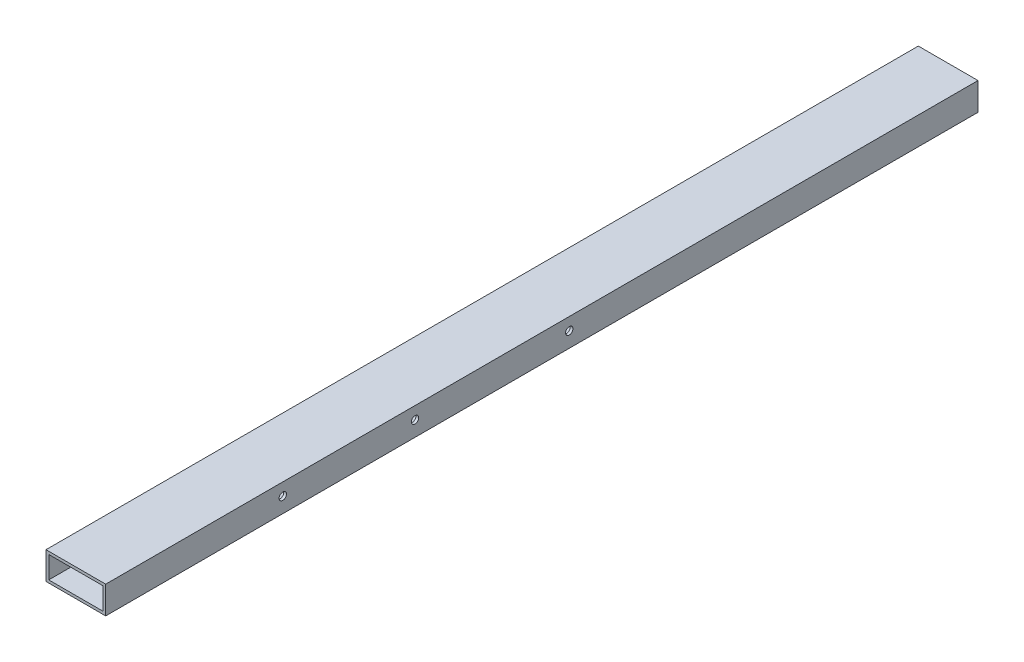
from build123d import *

# Parameters (mm, degrees)
SKETCH1_W           = 65
SKETCH1_H           = 30
BOSS_EXTRUDE1_DEPTH = 950
SKETCH2_W           = 59
SKETCH2_H           = 24
CUT_EXTRUDE1_DEPTH  = 950
SKETCH5_R           = 4
CUT_EXTRUDE2_DEPTH  = 954.05282071


with BuildPart() as part:
    # Sketch1 → Boss-Extrude1 (new body)
    with BuildSketch(Plane.XY):
        with Locations((-8.040751589, 24.808027615)):
            Rectangle(SKETCH1_W, SKETCH1_H)
    extrude(amount=BOSS_EXTRUDE1_DEPTH)

    # Sketch2 → Cut-Extrude1 (cut)
    with BuildSketch(Plane.XY.offset(950)):
        with Locations((-8.040751589, 24.808027615)):
            Rectangle(SKETCH2_W, SKETCH2_H)
    extrude(amount=-CUT_EXTRUDE1_DEPTH, mode=Mode.SUBTRACT)

    # Sketch5 → Cut-Extrude2 (cut, through all)
    with BuildSketch(Plane.ZY.offset(40.540751589)):
        with Locations((445.101574912, 26.308027615)):
            Circle(SKETCH5_R)
        with Locations((613.101574912, 26.308027615)):
            Circle(SKETCH5_R)
        with Locations((757.101574912, 26.308027615)):
            Circle(SKETCH5_R)
    extrude(amount=-CUT_EXTRUDE2_DEPTH, mode=Mode.SUBTRACT)


solid = part.part
